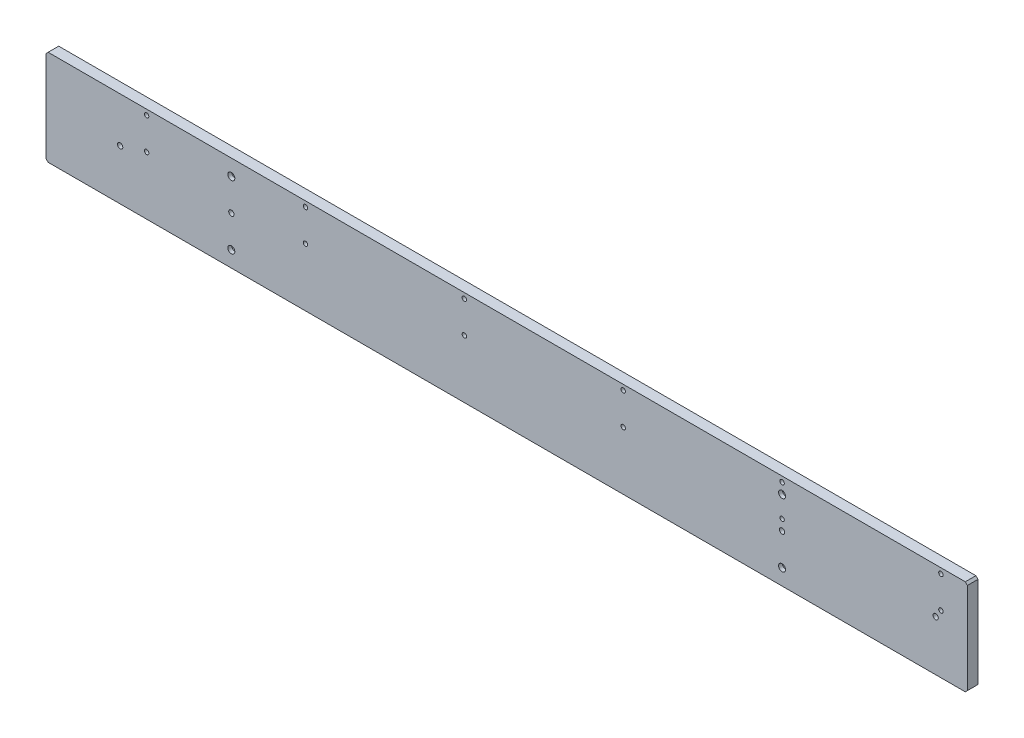
from build123d import *

# Parameters (mm, degrees)
SKETCH_1_W                   = 870
SKETCH_1_H                   = 90
EXTRUDE_1_DEPTH              = 10
CHAMFER_1_SIZE               = 2
HOLE_WIZARD_M6_1_D           = 6.6
HOLE_WIZARD_M6_1_CBORE_D     = 11
HOLE_WIZARD_M6_1_CBORE_DEPTH = 6.4
HOLE_WIZARD_5_0_5_1_D        = 5
HOLE_WIZARD_5_0_5_1_DEPTH    = 15.61
HOLE_WIZARD_5_0_5_1_TIP      = 1.443375673
SKETCH_8_R                   = 2.5
CUT_EXTRUDE_1_DEPTH          = 438.435709562
HOLE_WIZARD_M5_2_AT_2_COUNT  = 2
HOLE_WIZARD_M5_2_AT_2_PITCH  = 30
PATTERN_LINEAR_1_COUNT       = 6
PATTERN_LINEAR_1_PITCH       = 150
HOLE_WIZARD_M3_1_D           = 2.5
HOLE_WIZARD_M3_1_DEPTH       = 7.5
HOLE_WIZARD_M3_1_TIP         = 0.751075774


with BuildPart() as part:
    # 草图1 → 凸台-拉伸1 (new body)
    with BuildSketch(Plane.XY):
        Rectangle(SKETCH_1_W, SKETCH_1_H)
    extrude(amount=EXTRUDE_1_DEPTH)

    # 倒角1
    chamfer_1_edges = [part.edges().sort_by_distance(p)[0] for p in [
        (435, -45, 5),
        (-435, -45, 5),
        (-435, 45, 5),
        (435, 45, 5),
    ]]
    chamfer(chamfer_1_edges, length=CHAMFER_1_SIZE)

    # M6 六角凹头螺钉的柱形沉头孔1 (through all)
    with Locations(Plane(origin=(0, 0, 0), x_dir=(-1, 0, 0), z_dir=(0, 0, -1))):
        with Locations((-260, 30), (-260, -30), (260, -30), (260, 30), (-105.244391783, -69.250649642)):
            CounterBoreHole(HOLE_WIZARD_M6_1_D / 2, HOLE_WIZARD_M6_1_CBORE_D / 2, HOLE_WIZARD_M6_1_CBORE_DEPTH)

    # Ø5.0 (5) 直径孔1
    with Locations(Plane(origin=(0, 0, 0), x_dir=(-1, 0, 0), z_dir=(0, 0, -1))):
        with Locations((-260, 0), (260, 0)):
            Hole(HOLE_WIZARD_5_0_5_1_D / 2, depth=HOLE_WIZARD_5_0_5_1_DEPTH)
            with Locations((0, 0, -(HOLE_WIZARD_5_0_5_1_DEPTH + HOLE_WIZARD_5_0_5_1_TIP / 2))):  # 120° drill point
                Cone(0, HOLE_WIZARD_5_0_5_1_D / 2, HOLE_WIZARD_5_0_5_1_TIP, mode=Mode.SUBTRACT)

    # 草图8 → 切除-拉伸1 (cut, through all)
    with BuildSketch(Plane(origin=(0, 0, 0), x_dir=(-1, 0, 0), z_dir=(0, 0, -1))):
        with Locations((365, 2.5)):
            Circle(SKETCH_8_R)
        with Locations((-405, 2.5)):
            Circle(SKETCH_8_R)
    extrude(amount=-CUT_EXTRUDE_1_DEPTH, mode=Mode.SUBTRACT)

    # 草图9 → M5 螺纹孔2 (revolve, cut)
    with BuildSketch(Plane(origin=(410, 40, 10), x_dir=(0, -1, 0), z_dir=(1, 0, 0))):
        Polygon((0, 0), (0, 18.6618073), (2.1, 17.4), (2.1, 0), align=None)
    hole_wizard_m5_2 = revolve(axis=Axis((410, 40, 16.35), (0, 0, -1)), mode=Mode.SUBTRACT)

    # M5 螺纹孔2 at 2: M5 螺纹孔2 ×2
    with Locations(*[(0, -i * HOLE_WIZARD_M5_2_AT_2_PITCH, 0) for i in range(1, HOLE_WIZARD_M5_2_AT_2_COUNT)]):
        add(hole_wizard_m5_2, mode=Mode.SUBTRACT)

    # 阵列(线性)1: M5 螺纹孔2 ×6
    with Locations(*[(-i * PATTERN_LINEAR_1_PITCH, 0, 0) for i in range(1, PATTERN_LINEAR_1_COUNT)]):
        add(hole_wizard_m5_2, mode=Mode.SUBTRACT)

    # 阵列(线性)1 copy 1 sketch → 阵列(线性)1 copy 1 (revolve, cut)
    with BuildSketch(Plane(origin=(260, 10, 10), x_dir=(0, -1, 0), z_dir=(1, 0, 0))):
        Polygon((0, 0), (0, 18.6618073), (2.1, 17.4), (2.1, 0), align=None)
    revolve(axis=Axis((260, 10, 16.35), (0, 0, -1)), mode=Mode.SUBTRACT)

    # 阵列(线性)1 copy 2 sketch → 阵列(线性)1 copy 2 (revolve, cut)
    with BuildSketch(Plane(origin=(110, 10, 10), x_dir=(0, -1, 0), z_dir=(1, 0, 0))):
        Polygon((0, 0), (0, 18.6618073), (2.1, 17.4), (2.1, 0), align=None)
    revolve(axis=Axis((110, 10, 16.35), (0, 0, -1)), mode=Mode.SUBTRACT)

    # 阵列(线性)1 copy 3 sketch → 阵列(线性)1 copy 3 (revolve, cut)
    with BuildSketch(Plane(origin=(-40, 10, 10), x_dir=(0, -1, 0), z_dir=(1, 0, 0))):
        Polygon((0, 0), (0, 18.6618073), (2.1, 17.4), (2.1, 0), align=None)
    revolve(axis=Axis((-40, 10, 16.35), (0, 0, -1)), mode=Mode.SUBTRACT)

    # 阵列(线性)1 copy 4 sketch → 阵列(线性)1 copy 4 (revolve, cut)
    with BuildSketch(Plane(origin=(-190, 10, 10), x_dir=(0, -1, 0), z_dir=(1, 0, 0))):
        Polygon((0, 0), (0, 18.6618073), (2.1, 17.4), (2.1, 0), align=None)
    revolve(axis=Axis((-190, 10, 16.35), (0, 0, -1)), mode=Mode.SUBTRACT)

    # 阵列(线性)1 copy 5 sketch → 阵列(线性)1 copy 5 (revolve, cut)
    with BuildSketch(Plane(origin=(-340, 10, 10), x_dir=(0, -1, 0), z_dir=(1, 0, 0))):
        Polygon((0, 0), (0, 18.6618073), (2.1, 17.4), (2.1, 0), align=None)
    revolve(axis=Axis((-340, 10, 16.35), (0, 0, -1)), mode=Mode.SUBTRACT)

    # M3 螺纹孔1
    with Locations(Plane(origin=(0, 0, 0), x_dir=(-1, 0, 0), z_dir=(0, 0, -1))):
        with Locations((317, -16.4), (317, -40), (335, -40), (335, -16.4)):
            Hole(HOLE_WIZARD_M3_1_D / 2, depth=HOLE_WIZARD_M3_1_DEPTH)
            with Locations((0, 0, -(HOLE_WIZARD_M3_1_DEPTH + HOLE_WIZARD_M3_1_TIP / 2))):  # 118° drill point
                Cone(0, HOLE_WIZARD_M3_1_D / 2, HOLE_WIZARD_M3_1_TIP, mode=Mode.SUBTRACT)


solid = part.part
